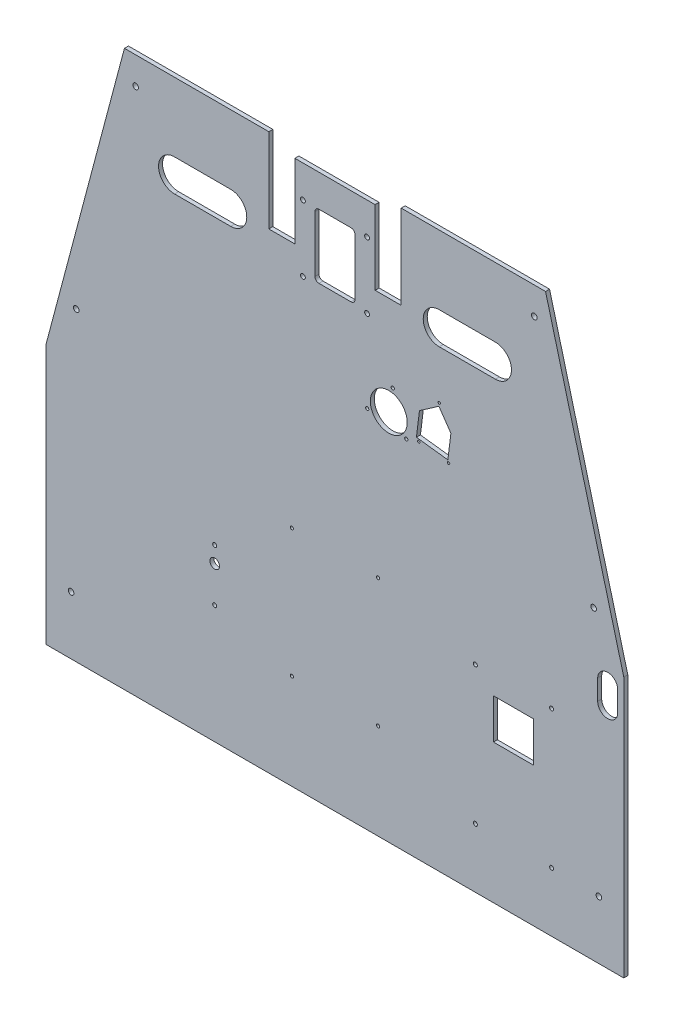
from build123d import *

# Parameters (mm, degrees)
BOSS_EXTRUDE1_DEPTH  = 10
SKETCH2_R            = 7
CUT_EXTRUDE1_DEPTH   = 10
LPATTERN1_COUNT      = 2
LPATTERN1_PITCH      = 1316
SKETCH3_R            = 7
CUT_EXTRUDE2_DEPTH   = 10
LPATTERN2_COUNT      = 2
LPATTERN2_PITCH      = 1290
SKETCH4_R            = 7
CUT_EXTRUDE3_DEPTH   = 10
LPATTERN3_COUNT      = 2
LPATTERN3_PITCH      = 994
CUT_EXTRUDE4_DEPTH   = 10
SKETCH6_W            = 100
SKETCH6_H            = 100
CUT_EXTRUDE5_DEPTH   = 10
SKETCH7_R            = 5
CUT_EXTRUDE6_DEPTH   = 10
LPATTERN4_COUNT      = 2
LPATTERN4_PITCH      = 190
LPATTERN4_COUNT_DIR2 = 2
LPATTERN4_PITCH_DIR2 = 344
SKETCH8_R            = 4
CUT_EXTRUDE7_DEPTH   = 10
LPATTERN5_COUNT      = 2
LPATTERN5_PITCH      = 320
LPATTERN5_COUNT_DIR2 = 2
LPATTERN5_PITCH_DIR2 = 215
CUT_EXTRUDE8_DEPTH   = 10
LPATTERN6_COUNT      = 2
LPATTERN6_PITCH      = 660
SKETCH10_W           = 100
SKETCH10_H           = 160
CUT_EXTRUDE9_DEPTH   = 10
FILLET1_R            = 10
SKETCH11_R           = 6
CUT_EXTRUDE10_DEPTH  = 10
LPATTERN7_COUNT      = 2
LPATTERN7_PITCH      = 160
LPATTERN7_COUNT_DIR2 = 2
LPATTERN7_PITCH_DIR2 = 165
SKETCH12_R           = 4
CUT_EXTRUDE11_DEPTH  = 10
SKETCH14_R           = 46
CUT_EXTRUDE12_DEPTH  = 10
SKETCH15_R           = 4
CUT_EXTRUDE13_DEPTH  = 10
LPATTERN8_COUNT      = 2
LPATTERN8_PITCH      = 99
SKETCH16_R           = 3
CUT_EXTRUDE14_DEPTH  = 10
CUT_EXTRUDE15_DEPTH  = 10
SKETCH18_R           = 3
CUT_EXTRUDE16_DEPTH  = 10
LPATTERN9_COUNT      = 2
LPATTERN9_PITCH      = 75
SKETCH19_R           = 5
CUT_EXTRUDE17_DEPTH  = 10
LPATTERN10_COUNT     = 2
LPATTERN10_PITCH     = 130
SKETCH20_R           = 12
CUT_EXTRUDE18_DEPTH  = 10
SKETCH21_W           = 65
SKETCH21_H           = 210
CUT_EXTRUDE19_DEPTH  = 10
SKETCH22_W           = 65
SKETCH22_H           = 210
CUT_EXTRUDE20_DEPTH  = 10
SKETCH23_W           = 200
SKETCH23_H           = 25
CUT_EXTRUDE21_DEPTH  = 10


with BuildPart() as part:
    # Sketch1 → Boss-Extrude1 (new body)
    with BuildSketch(Plane.XY):
        Polygon((-720, 0), (720, 0), (720, 650), (525, 1385), (-525, 1385), (-720, 650), align=None)
    extrude(amount=BOSS_EXTRUDE1_DEPTH)

    # Sketch2 → Cut-Extrude1 (cut)
    with BuildSketch(Plane.XY.offset(10)):
        with Locations((-658, 145)):
            Circle(SKETCH2_R)
    cut_extrude1 = extrude(amount=-CUT_EXTRUDE1_DEPTH, mode=Mode.SUBTRACT)

    # LPattern1: Cut-Extrude1 ×2
    with Locations(*[(i * LPATTERN1_PITCH, 0, 0) for i in range(1, LPATTERN1_COUNT)]):
        add(cut_extrude1, mode=Mode.SUBTRACT)

    # Sketch3 → Cut-Extrude2 (cut)
    with BuildSketch(Plane.XY.offset(10)):
        with Locations((-645, 762)):
            Circle(SKETCH3_R)
    cut_extrude2 = extrude(amount=-CUT_EXTRUDE2_DEPTH, mode=Mode.SUBTRACT)

    # LPattern2: Cut-Extrude2 ×2
    with Locations(*[(i * LPATTERN2_PITCH, 0, 0) for i in range(1, LPATTERN2_COUNT)]):
        add(cut_extrude2, mode=Mode.SUBTRACT)

    # Sketch4 → Cut-Extrude3 (cut)
    with BuildSketch(Plane.XY.offset(10)):
        with Locations((-497, 1317)):
            Circle(SKETCH4_R)
    cut_extrude3 = extrude(amount=-CUT_EXTRUDE3_DEPTH, mode=Mode.SUBTRACT)

    # LPattern3: Cut-Extrude3 ×2
    with Locations(*[(i * LPATTERN3_PITCH, 0, 0) for i in range(1, LPATTERN3_COUNT)]):
        add(cut_extrude3, mode=Mode.SUBTRACT)

    # Sketch5 → Cut-Extrude4 (cut)
    with BuildSketch(Plane.XY.offset(10)):
        with BuildLine():
            Line((655, 615), (655, 565))
            ThreePointArc((655, 565), (680, 540), (705, 565))
            Line((705, 565), (705, 615))
            ThreePointArc((705, 615), (680, 640), (655, 615))
        make_face()
    extrude(amount=-CUT_EXTRUDE4_DEPTH, mode=Mode.SUBTRACT)

    # Sketch6 → Cut-Extrude5 (cut)
    with BuildSketch(Plane.XY.offset(10)):
        with Locations((445, 397)):
            Rectangle(SKETCH6_W, SKETCH6_H)
    extrude(amount=-CUT_EXTRUDE5_DEPTH, mode=Mode.SUBTRACT)

    # Sketch7 → Cut-Extrude6 (cut)
    with BuildSketch(Plane.XY.offset(10)):
        with Locations((540, 492)):
            Circle(SKETCH7_R)
    cut_extrude6 = extrude(amount=-CUT_EXTRUDE6_DEPTH, mode=Mode.SUBTRACT)

    # LPattern4: Cut-Extrude6 2 × 2
    with Locations(*[(-i * LPATTERN4_PITCH, -j * LPATTERN4_PITCH_DIR2, 0) for i in range(LPATTERN4_COUNT) for j in range(LPATTERN4_COUNT_DIR2) if (i, j) != (0, 0)]):
        add(cut_extrude6, mode=Mode.SUBTRACT)

    # Sketch8 → Cut-Extrude7 (cut)
    with BuildSketch(Plane.XY.offset(10)):
        with Locations((107.5, 238)):
            Circle(SKETCH8_R)
    cut_extrude7 = extrude(amount=-CUT_EXTRUDE7_DEPTH, mode=Mode.SUBTRACT)

    # LPattern5: Cut-Extrude7 2 × 2
    with Locations(*[(-j * LPATTERN5_PITCH_DIR2, i * LPATTERN5_PITCH, 0) for i in range(LPATTERN5_COUNT) for j in range(LPATTERN5_COUNT_DIR2) if (i, j) != (0, 0)]):
        add(cut_extrude7, mode=Mode.SUBTRACT)

    # Sketch9 → Cut-Extrude8 (cut)
    with BuildSketch(Plane.XY.offset(10)):
        with BuildLine():
            Line((-400, 1133), (-260, 1133))
            ThreePointArc((-260, 1133), (-220, 1173), (-260, 1213))
            Line((-260, 1213), (-400, 1213))
            ThreePointArc((-400, 1213), (-440, 1173), (-400, 1133))
        make_face()
    cut_extrude8 = extrude(amount=-CUT_EXTRUDE8_DEPTH, mode=Mode.SUBTRACT)

    # LPattern6: Cut-Extrude8 ×2
    with Locations(*[(i * LPATTERN6_PITCH, 0, 0) for i in range(1, LPATTERN6_COUNT)]):
        add(cut_extrude8, mode=Mode.SUBTRACT)

    # Sketch10 → Cut-Extrude9 (cut)
    with BuildSketch(Plane.XY.offset(10)):
        with Locations((0, 1200)):
            Rectangle(SKETCH10_W, SKETCH10_H)
    extrude(amount=-CUT_EXTRUDE9_DEPTH, mode=Mode.SUBTRACT)

    # Fillet1
    fillet1_edges = [part.edges().sort_by_distance(p)[0] for p in [
        (-50, 1120, 5),
        (-50, 1280, 5),
        (50, 1280, 5),
        (50, 1120, 5),
    ]]
    fillet(fillet1_edges, radius=FILLET1_R)

    # Sketch11 → Cut-Extrude10 (cut)
    with BuildSketch(Plane.XY.offset(10)):
        with Locations((80, 1280)):
            Circle(SKETCH11_R)
    cut_extrude10 = extrude(amount=-CUT_EXTRUDE10_DEPTH, mode=Mode.SUBTRACT)

    # LPattern7: Cut-Extrude10 2 × 2
    with Locations(*[(-i * LPATTERN7_PITCH, -j * LPATTERN7_PITCH_DIR2, 0) for i in range(LPATTERN7_COUNT) for j in range(LPATTERN7_COUNT_DIR2) if (i, j) != (0, 0)]):
        add(cut_extrude10, mode=Mode.SUBTRACT)

    # Sketch12 → Cut-Extrude11 (cut)
    with BuildSketch(Plane.XY.offset(10)):
        with Locations((144, 986)):
            Circle(SKETCH12_R)
    extrude(amount=-CUT_EXTRUDE11_DEPTH, mode=Mode.SUBTRACT)

    # Sketch14 → Cut-Extrude12 (cut)
    with BuildSketch(Plane.XY.offset(10)):
        with Locations((134.067324237, 929.668996528)):
            Circle(SKETCH14_R)
    extrude(amount=-CUT_EXTRUDE12_DEPTH, mode=Mode.SUBTRACT)

    # Sketch15 → Cut-Extrude13 (cut)
    with BuildSketch(Plane.XY.offset(10)):
        with Locations((80.318272947, 909.902118035)):
            Circle(SKETCH15_R)
    cut_extrude13 = extrude(amount=-CUT_EXTRUDE13_DEPTH, mode=Mode.SUBTRACT)

    # LPattern8: Cut-Extrude13 ×2
    with Locations(*[Vector(0.9848077530122089, -0.17364817766692592, 0) * (i * LPATTERN8_PITCH) for i in range(1, LPATTERN8_COUNT)]):
        add(cut_extrude13, mode=Mode.SUBTRACT)

    # Sketch16 → Cut-Extrude14 (cut)
    with BuildSketch(Plane.XY.offset(10)):
        with Locations((260, 1012)):
            Circle(SKETCH16_R)
    extrude(amount=-CUT_EXTRUDE14_DEPTH, mode=Mode.SUBTRACT)

    # Sketch17 → Cut-Extrude15 (cut)
    with BuildSketch(Plane.XY.offset(10)):
        Polygon((259.025045253, 1004.059630787), (210.570516199, 970.471558288), (203.044210897, 909.174720581), (281.455356876, 899.547042452), (288.981662179, 960.843880159), align=None)
    extrude(amount=-CUT_EXTRUDE15_DEPTH, mode=Mode.SUBTRACT)

    # Sketch18 → Cut-Extrude16 (cut)
    with BuildSketch(Plane.XY.offset(10)):
        with Locations((208.764544822, 902.427292939)):
            Circle(SKETCH18_R)
    cut_extrude16 = extrude(amount=-CUT_EXTRUDE16_DEPTH, mode=Mode.SUBTRACT)

    # LPattern9: Cut-Extrude16 ×2
    with Locations(*[Vector(0.9925461516413229, -0.121869343405141, 0) * (i * LPATTERN9_PITCH) for i in range(1, LPATTERN9_COUNT)]):
        add(cut_extrude16, mode=Mode.SUBTRACT)

    # Sketch19 → Cut-Extrude17 (cut)
    with BuildSketch(Plane.XY.offset(10)):
        with Locations((-300, 295)):
            Circle(SKETCH19_R)
    cut_extrude17 = extrude(amount=-CUT_EXTRUDE17_DEPTH, mode=Mode.SUBTRACT)

    # LPattern10: Cut-Extrude17 ×2
    with Locations(*[(0, i * LPATTERN10_PITCH, 0) for i in range(1, LPATTERN10_COUNT)]):
        add(cut_extrude17, mode=Mode.SUBTRACT)

    # Sketch20 → Cut-Extrude18 (cut)
    with BuildSketch(Plane.XY.offset(10)):
        with Locations((-300, 385)):
            Circle(SKETCH20_R)
    extrude(amount=-CUT_EXTRUDE18_DEPTH, mode=Mode.SUBTRACT)

    # Sketch21 → Cut-Extrude19 (cut)
    with BuildSketch(Plane.XY.offset(10)):
        with Locations((132.5, 1280)):
            Rectangle(SKETCH21_W, SKETCH21_H)
    extrude(amount=-CUT_EXTRUDE19_DEPTH, mode=Mode.SUBTRACT)

    # Sketch22 → Cut-Extrude20 (cut)
    with BuildSketch(Plane.XY.offset(10)):
        with Locations((-132.5, 1280)):
            Rectangle(SKETCH22_W, SKETCH22_H)
    extrude(amount=-CUT_EXTRUDE20_DEPTH, mode=Mode.SUBTRACT)

    # Sketch23 → Cut-Extrude21 (cut)
    with BuildSketch(Plane.XY.offset(10)):
        with Locations((0, 1372.5)):
            Rectangle(SKETCH23_W, SKETCH23_H)
    extrude(amount=-CUT_EXTRUDE21_DEPTH, mode=Mode.SUBTRACT)


solid = part.part
